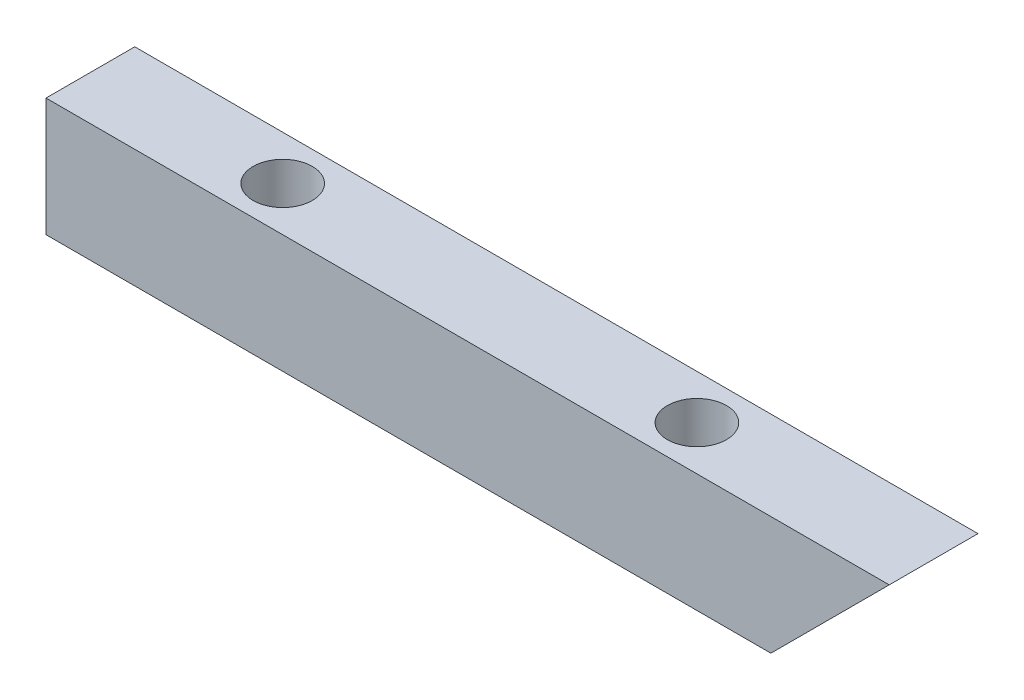
from build123d import *

# Parameters (mm, degrees)
SKETCH_1_W          = 270
SKETCH_1_H          = 30
EXTRUDE_1_DEPTH     = 40
SKETCH_2_R          = 10
CUT_EXTRUDE_2_DEPTH = 30
SKETCH_3_W          = 30
SKETCH_3_H          = 40
EXTRUDE_2_DEPTH     = 15
CUT_EXTRUDE_3_DEPTH = 159.113883008


with BuildPart() as part:
    # 草图1 → 凸台-拉伸1 (new body)
    with BuildSketch(Plane(origin=(0, 0, 0), x_dir=(1, 0, 0), z_dir=(0, 1, 0))):
        Rectangle(SKETCH_1_W, SKETCH_1_H)
    extrude(amount=EXTRUDE_1_DEPTH)

    # 草图2 → 切除-拉伸2 (cut)
    with BuildSketch(Plane(origin=(0, 40, 0), x_dir=(1, 0, 0), z_dir=(0, 1, 0))):
        with Locations(Location((70, 0, 0), (0, 0, 270))):
            Circle(SKETCH_2_R)
        with Locations(Location((-70, 0, 0), (0, 0, 90))):
            Circle(SKETCH_2_R)
    extrude(amount=-CUT_EXTRUDE_2_DEPTH, mode=Mode.SUBTRACT)

    # 草图3 → 凸台-拉伸2 (add)
    with BuildSketch(Plane(origin=(135, 0, 0), x_dir=(0, 0, -1), z_dir=(1, 0, 0))):
        with Locations((0, 20)):
            Rectangle(SKETCH_3_W, SKETCH_3_H)
    extrude(amount=EXTRUDE_2_DEPTH)

    # 草图4 → 切除-拉伸3 (cut, through all)
    with BuildSketch(Plane.XY.offset(15)):
        Polygon((150, 40), (110, 0), (150, 0), align=None)
    extrude(amount=-CUT_EXTRUDE_3_DEPTH, mode=Mode.SUBTRACT)


solid = part.part
